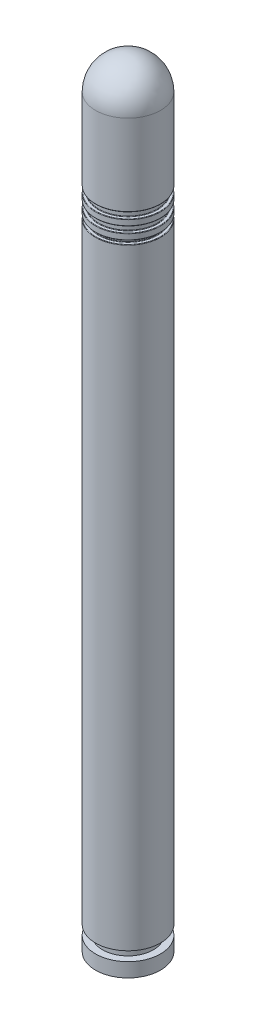
SolidWorks part; units mm, degrees
material "ABS"
ref_plane "Front Plane" through (0, 0, 0) normal (0, 0, 1) x (1, 0, 0)
ref_plane "Top Plane" through (0, 0, 0) normal (0, 1, 0) x (1, 0, 0)
ref_plane "Right Plane" through (0, 0, 0) normal (1, 0, 0) x (0, 0, -1)
sketch "Sketch1" plane through (0, 0, 0) normal (0, 0, 1) x (1, 0, 0)
  line L0 (0, -7.8737) -> (0, 95.773) construction
  line L1 (2, 0.2) -> (3.45, 0.2)
  line L2 (3.45, 0.2) -> (3.45, 1.7)
  line L3 (3.45, 2.7) -> (2.7, 2.7)
  line L4 (2.7, 2.7) -> (2.7, 1.7)
  line L5 (2.7, 1.7) -> (3.45, 1.7)
  line L6 (3.45, 2.7) -> (3.45, 67.65)
  line L7 (3.15, 67.7) -> (3.4, 67.7)
  line L8 (3.15, 70.7) -> (3.4, 70.7)
  line L9 (3.1, 70.65) -> (3.1, 70.1)
  line L10 (3.15, 70.05) -> (3.4, 70.05)
  line L11 (3.15, 69.4) -> (3.4, 69.4)
  line L12 (3.15, 68.75) -> (3.4, 68.75)
  line L13 (3.15, 68.1) -> (3.4, 68.1)
  line L14 (3.45, 70.75) -> (3.45, 79.35)
  line L15 (3.45, 68.15) -> (3.45, 68.7)
  line L16 (3.45, 69.45) -> (3.45, 70)
  line L17 (3.1, 68.05) -> (3.1, 67.75)
  line L18 (3.1, 69.35) -> (3.1, 68.8)
  line L19 (0, 70.7) -> (3.45, 70.7) construction
  line L20 (0, 67.7) -> (3.45, 67.7) construction
  line L21 (2, 0.2) -> (2, 79.35)
  line L22 (2, 79.35) -> (0, 79.35)
  line L23 (0, 79.35) -> (0, 82.8)
  line L24 (0, 0.2) -> (3.45, 0.2) construction
  arc A0 (3.45, 79.35) -> (0, 82.8) centre (0, 79.35) ccw
  arc A1 (3.4, 67.7) -> (3.45, 67.65) centre (3.4, 67.65) cw
  arc A2 (3.15, 67.7) -> (3.1, 67.75) centre (3.15, 67.75) cw
  arc A3 (3.15, 68.1) -> (3.1, 68.05) centre (3.15, 68.05) ccw
  arc A4 (3.4, 68.1) -> (3.45, 68.15) centre (3.4, 68.15) ccw
  arc A5 (3.4, 68.75) -> (3.45, 68.7) centre (3.4, 68.7) cw
  arc A6 (3.15, 68.75) -> (3.1, 68.8) centre (3.15, 68.8) cw
  arc A7 (3.15, 69.4) -> (3.1, 69.35) centre (3.15, 69.35) ccw
  arc A8 (3.4, 69.4) -> (3.45, 69.45) centre (3.4, 69.45) ccw
  arc A9 (3.4, 70.05) -> (3.45, 70) centre (3.4, 70) cw
  arc A10 (3.15, 70.05) -> (3.1, 70.1) centre (3.15, 70.1) cw
  arc A11 (3.4, 70.7) -> (3.45, 70.75) centre (3.4, 70.75) ccw
  arc A12 (3.1, 70.65) -> (3.15, 70.7) centre (3.15, 70.65) cw
  point P33 (3.1, 68.1)
  point P42 (3.1, 69.4)
  dimension "D1" = 6.9
  dimension "D10" = 0.05
  dimension "D2" = 82.6
  dimension "D3" = 1.5
  dimension "D4" = 1
  dimension "D5" = 5.4
  dimension "D8" = 6.2
  dimension "D11" = 4
  dimension "D6" = 67.5
  dimension "D7" = 3
  dimension "D9" = 5
revolve "Revolve1" add sketch "Sketch1" angle 360 about L0
